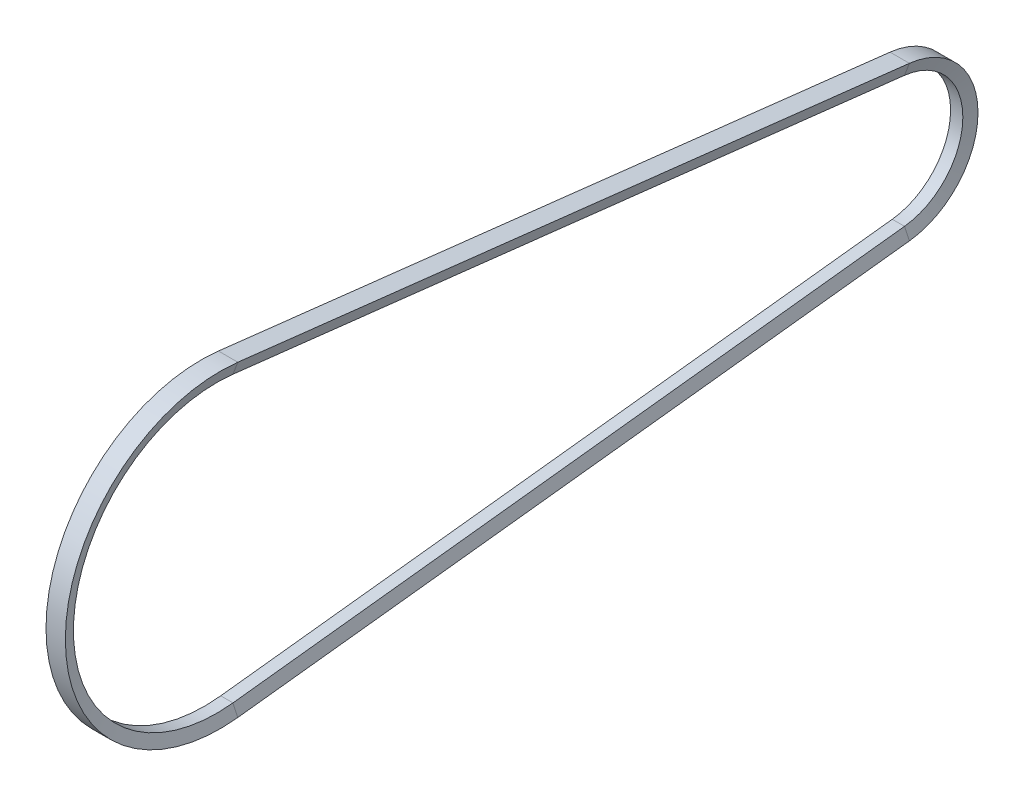
SolidWorks part; units mm, degrees
ref_plane "前视基准面" through (0, 0, 0) normal (0, 0, 1) x (1, 0, 0)
ref_plane "上视基准面" through (0, 0, 0) normal (0, 1, 0) x (1, 0, 0)
ref_plane "右视基准面" through (0, 0, 0) normal (1, 0, 0) x (0, 0, -1)
sketch "草图1" plane through (0, 0, 0) normal (1, 0, 0) x (0, 0, -1)
  line L0 (9.1038, 79.4803) -> (356.0519, 39.7402)
  line L1 (9.1038, -79.4803) -> (356.0519, -39.7402)
  line L2 (0, 0) -> (351.5, 0) construction
  arc A0 (9.1038, 79.4803) -> (9.1038, -79.4803) centre (0, 0) ccw
  arc A1 (356.0519, -39.7402) -> (356.0519, 39.7402) centre (351.5, 0) ccw
sketch "草图2" plane through (0, 0, 0) normal (0, 0, 1) x (1, 0, 0)
  line L0 (-5, 80) -> (5, 80)
  line L1 (5, 80) -> (3.1656, 74)
  line L2 (3.1656, 74) -> (-3.1656, 74)
  line L3 (-3.1656, 74) -> (-5, 80)
  line L4 (0, 74) -> (0, 80) construction
  line L5 (0, -80) -> (0, 80) construction
sweep "扫描1" add profiles "草图2" path "草图1"
equation "\"D3@草图1\" = \"D1@距离1@实心轮_辐板轮.SLDASM\""
equation "\"D1@草图2\"=10mm"
equation "\"D2@草图2\"=6mm"
equation "\"D3@草图2\" = \"槽轮角@草图1@大带轮_辐板轮<1>.Part\""
equation "\"D2@草图1\" = \"dd@草图1@小带轮_实心轮<1>.Part\" / 2"
equation "\"D1@草图1\" = \"dd@草图1@大带轮_辐板轮<1>.Part\" / 2"
